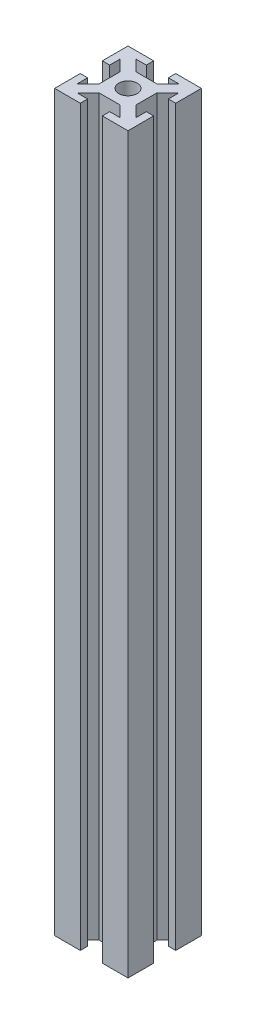
from build123d import *

# Parameters (mm, degrees)
SKETCH1_R           = 5
BOSS_EXTRUDE1_DEPTH = 400


with BuildPart() as part:
    # Sketch1 → Boss-Extrude1 (new body)
    with BuildSketch(Plane(origin=(0, 0, 0), x_dir=(1, 0, 0), z_dir=(0, 1, 0))):
        Polygon((-6, 20), (-6, 16), (-11.757359313, 16), (-5.757359313, 10), (5.757359313, 10), (11.757359313, 16), (6, 16), (6, 20), (20, 20), (20, 6), (16, 6), (16, 11.757359313), (10, 5.757359313), (10, -5.757359313), (16, -11.757359313), (16, -6), (20, -6), (20, -20), (6, -20), (6, -16), (11.757359313, -16), (5.757359313, -10), (-5.757359313, -10), (-11.757359313, -16), (-6, -16), (-6, -20), (-20, -20), (-20, -6), (-16, -6), (-16, -11.757359313), (-10, -5.757359313), (-10, 5.757359313), (-16, 11.757359313), (-16, 6), (-20, 6), (-20, 20), align=None)
        with Locations(Location((0, 0, 0), (0, 0, 270))):
            Circle(SKETCH1_R, mode=Mode.SUBTRACT)
    extrude(amount=BOSS_EXTRUDE1_DEPTH)


solid = part.part
